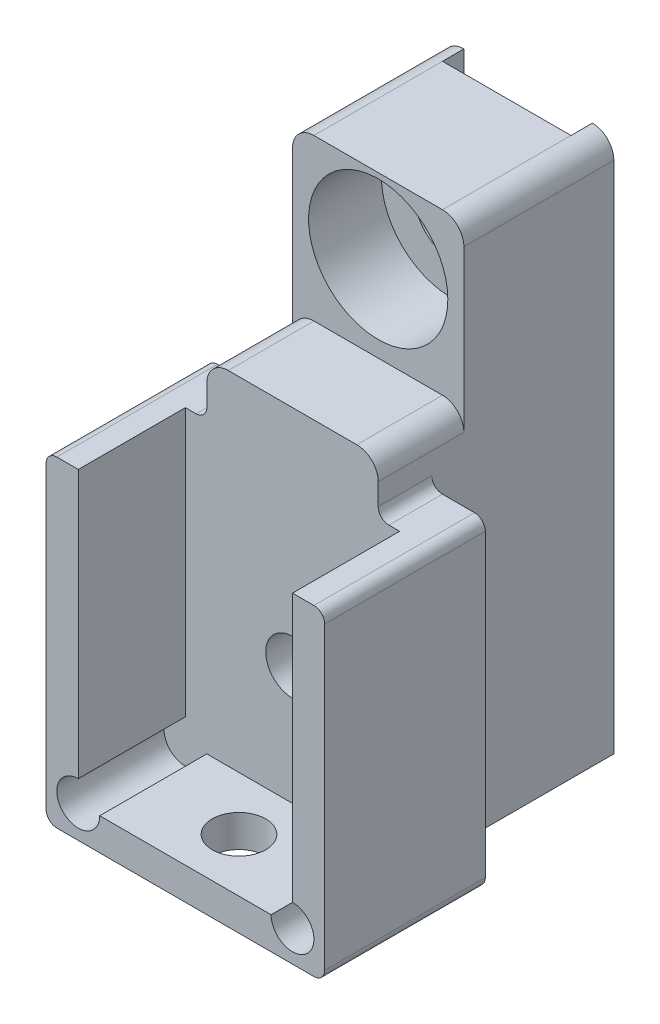
SolidWorks part; units mm, degrees
material "S136"
ref_plane "Front Plane" through (0, 0, 0) normal (0, 0, 1) x (1, 0, 0)
ref_plane "Top Plane" through (0, 0, 0) normal (0, 1, 0) x (1, 0, 0)
ref_plane "Right Plane" through (0, 0, 0) normal (1, 0, 0) x (0, 0, -1)
sketch "Sketch1" plane through (0, 0, 0) normal (0, 0, 1) x (1, 0, 0)
  line L1 (-6.5, 12.5) -> (6.5, 12.5)
  line L2 (-6.5, 12.5) -> (-6.5, -12.5)
  line L3 (-6.5, -12.5) -> (6.5, -12.5)
  line L4 (6.5, 12.5) -> (6.5, -12.5)
  line L5 (-6.5, 12.5) -> (6.5, -12.5) construction
  line L6 (-6.5, -12.5) -> (6.5, 12.5) construction
  point P0 (0, 0)
  dimension "13" = 13
  dimension "D2" = 25
extrude "Boss-Extrude1" add sketch "Sketch1" along normal blind 10
sketch "Sketch2" plane through (0, 0, 10) normal (0, 0, 1) x (1, 0, 0)
  line L0 (0, 0) -> (0, -5.4615) construction
  line L1 (-6.5, 12.5) -> (-4, 12.5)
  line L2 (-6.5, 12.5) -> (-6.5, 2.5)
  line L3 (-6.5, 2.5) -> (-4, 2.5)
  line L4 (-4, 12.5) -> (-4, 2.5)
  line L5 (4, 12.5) -> (4, 2.5)
  line L6 (6.5, 2.5) -> (4, 2.5)
  line L7 (6.5, 12.5) -> (6.5, 2.5)
  line L8 (6.5, 12.5) -> (4, 12.5)
  dimension "D1" = 4
  dimension "D2" = 10
extrude "Cut-Extrude1" cut sketch "Sketch2" against normal through all both and the other way through all
fillet "Fillet1" radius 0.5 6 edges at (4, 2.5, 5) (-4, 2.5, 5) (6.5, 2.5, 5) (6.5, -12.5, 5) (-6.5, -12.5, 5) (-6.5, 2.5, 5)
fillet "Fillet2" radius 1 2 edges at (4, 12.5, 5) (-4, 12.5, 5)
sketch "Sketch8" plane through (0, 0, 0) normal (0, 0, -1) x (-1, 0, 0)
  line L0 (-3, 12.5) -> (3, 12.5) construction
  line L1 (-3, -20.0892) -> (3, -20.0892)
  line L2 (-3, -20.0892) -> (-3, 12.5)
  line L3 (-3, 12.5) -> (3, 12.5)
  line L4 (3, -20.0892) -> (3, 12.5)
  line L5 (-3, -20.0892) -> (3, 12.5) construction
  line L6 (-3, 12.5) -> (3, -20.0892) construction
  line L7 (0, 0) -> (0, 24.6616) construction
  point P0 (0, -3.7946)
  dimension "D1" = 6
extrude "Cut-Extrude4" cut sketch "Sketch8" against normal blind 1
sketch "Sketch21" plane through (0, 0, 10) normal (0, 0, 1) x (1, 0, 0)
  line L0 (-6, -12.5) -> (6, -12.5) construction
  line L1 (-5, 19.6027) -> (5, 19.6027)
  line L2 (-5, 19.6027) -> (-5, -11)
  line L3 (-5, -11) -> (5, -11)
  line L4 (5, 19.6027) -> (5, -11)
  line L5 (6.5, -12) -> (6.5, 2) construction
  line L6 (-6.5, 2) -> (-6.5, -12) construction
  dimension "D1" = 1.5
  dimension "D2" = 1.5
  dimension "D3" = 1.5
extrude "Cut-Extrude11" cut sketch "Sketch21" against normal blind 1
sketch "Sketch25" plane through (0, 0, 9) normal (0, 0, 1) x (1, 0, 0)
  line L0 (3, 12.5) -> (-3, 12.5) construction
  line L1 (-8.1526, 20.6765) -> (5.6484, 20.6765)
  line L2 (-8.1526, 20.6765) -> (-8.1526, 5)
  line L3 (-8.1526, 5) -> (5.6484, 5)
  line L4 (5.6484, 20.6765) -> (5.6484, 5)
  dimension "D1" = 7.5
extrude "Cut-Extrude13" cut sketch "Sketch25" against normal blind 2
fillet "Fillet3" radius 1 2 edges at (4, 5, 8) (-4, 5, 8)
hole_wizard "CBORE for M3 Hex Socket Head Cap Screw2" positions "Sketch26" profile "Sketch27" counterbore size "M3" standard "ISO" end condition up to next
sketch "Sketch26" plane through (0, 0, 9) normal (0, 0, 1) x (1, 0, 0)
  line L0 (3, 12.5) -> (-3, 12.5) construction
  point P0 (0, 9)
  dimension "D2" = 3.5
sketch "Sketch27" plane through (0, 9, 9) normal (1, 0, 0) x (0, -1, 0)
  line L0 (0, 0) -> (0, 8)
  line L1 (0, 8) -> (1.7, 8)
  line L3 (1.7, 8) -> (1.7, 5.4)
  line L4 (1.7, 5.4) -> (3.25, 5.4)
  line L5 (3.25, 5.4) -> (3.25, 0)
  line L7 (3.25, 0) -> (0, 0)
  line L11 (0, -6.35) -> (0, 107.95) construction
  dimension "通孔孔直径" = 3.4
  dimension "通孔孔深度" = 8
  dimension "柱形沉头孔直径" = 6.5
  dimension "柱形沉头孔深度" = 5.4
sketch "Sketch31" plane through (0, 0, 10) normal (0, 0, 1) x (1, 0, 0)
  line L8 (-5, -11) -> (-5, 2.5)
  line L9 (-5, 2.5) -> (-6, 2.5)
  line L10 (-6.5, 2) -> (-6.5, -12)
  line L11 (-6, -12.5) -> (6, -12.5)
  line L12 (6.5, -12) -> (6.5, 2)
  line L13 (6, 2.5) -> (5, 2.5)
  line L15 (-5, -11) -> (-5, 2.5)
  line L17 (-5, 2.5) -> (-6, 2.5)
  line L18 (-6.5, 2) -> (-6.5, -12)
  line L19 (-6, -12.5) -> (6, -12.5)
  line L20 (6.5, -12) -> (6.5, 2)
  line L21 (6, 2.5) -> (5, 2.5)
  line L25 (5, 2.5) -> (5, -11)
  line L27 (5, 2.5) -> (5, -11)
  line L28 (5, -11) -> (-5, -11)
  line L29 (5, -11) -> (-5, -11)
  arc A6 (-6, 2.5) -> (-6.5, 2) centre (-6, 2) ccw
  arc A7 (-6.5, -12) -> (-6, -12.5) centre (-6, -12) ccw
  arc A8 (6, -12.5) -> (6.5, -12) centre (6, -12) ccw
  arc A9 (6.5, 2) -> (6, 2.5) centre (6, 2) ccw
  arc A12 (-6, 2.5) -> (-6.5, 2) centre (-6, 2) ccw
  arc A13 (-6.5, -12) -> (-6, -12.5) centre (-6, -12) ccw
  arc A14 (6, -12.5) -> (6.5, -12) centre (6, -12) ccw
  arc A15 (6.5, 2) -> (6, 2.5) centre (6, 2) ccw
  dimension "D1" = 0
extrude "Boss-Extrude4" add sketch "Sketch31" along normal blind 6
sketch "Sketch33" plane through (-6.5, 0, 0) normal (-1, 0, 0) x (0, 0, 1)
  line L0 (1, 12.5) -> (7, 12.5) construction
  line L1 (-1.8788, 3.5) -> (8.5, 3.5)
  line L2 (-1.8788, 3.5) -> (-1.8788, -16.5)
  line L3 (-1.8788, -16.5) -> (8.5, -16.5)
  line L4 (8.5, 3.5) -> (8.5, -16.5)
  line L5 (0, 3) -> (0, 11.5) construction
  dimension "D1" = 8.5
  dimension "D2" = 9
  dimension "D3" = 20
extrude "Cut-Extrude15" cut sketch "Sketch33" against normal up to surface (2.5 mm away) up to face at (-4, 6.1667, 5.3333)
sketch "Sketch34" plane through (6.5, 0, 0) normal (1, 0, 0) x (0, 0, -1)
  line L0 (0, -12) -> (0, 2) construction
  line L1 (-8.5, -16.2363) -> (1.421, -16.2363)
  line L2 (-8.5, -16.2363) -> (-8.5, 3.5)
  line L3 (-8.5, 3.5) -> (1.421, 3.5)
  line L4 (1.421, -16.2363) -> (1.421, 3.5)
  line L5 (-7, 12.5) -> (-1, 12.5) construction
  dimension "D1" = 8.5
  dimension "D2" = 9
extrude "Cut-Extrude16" cut sketch "Sketch34" against normal up to surface (2.5 mm away) up to face at (4, 6.1667, 5.3333)
sketch "Sketch36" plane through (0, 0, 9) normal (0, 0, 1) x (1, 0, 0)
  line L8 (-5, 2.5) -> (-5, -11)
  line L9 (-5, -11) -> (5, -11)
  line L10 (5, -11) -> (5, 2.5)
  line L11 (5, 2.5) -> (4.5, 2.5)
  line L12 (4, 3) -> (4, 4)
  line L13 (3, 5) -> (-3, 5)
  line L14 (-4, 4) -> (-4, 3)
  line L15 (-4.5, 2.5) -> (-5, 2.5)
  line L16 (-5, 2.5) -> (-5, -11)
  line L17 (-5, -11) -> (5, -11)
  line L18 (5, -11) -> (5, 2.5)
  line L19 (5, 2.5) -> (4.5, 2.5)
  line L20 (4, 3) -> (4, 4)
  line L21 (3, 5) -> (-3, 5)
  line L22 (-4, 4) -> (-4, 3)
  line L23 (-4.5, 2.5) -> (-5, 2.5)
  arc A8 (4, 3) -> (4.5, 2.5) centre (4.5, 3) ccw
  arc A9 (4, 4) -> (3, 5) centre (3, 4) ccw
  arc A10 (-3, 5) -> (-4, 4) centre (-3, 4) ccw
  arc A11 (-4.5, 2.5) -> (-4, 3) centre (-4.5, 3) ccw
  arc A14 (4, 3) -> (4.5, 2.5) centre (4.5, 3) ccw
  arc A15 (4, 4) -> (3, 5) centre (3, 4) ccw
  arc A16 (-3, 5) -> (-4, 4) centre (-3, 4) ccw
  arc A17 (-4.5, 2.5) -> (-4, 3) centre (-4.5, 3) ccw
  dimension "D1" = 0
extrude "Boss-Extrude5" add sketch "Sketch36" along normal blind 2
hole_wizard "M3 Tapped Hole1" positions "Sketch37" profile "Sketch38" tap size "M3" standard "ISO"
sketch "Sketch37" plane through (0, 0, 11) normal (0, 0, 1) x (1, 0, 0)
  line L0 (-6, -12.5) -> (6, -12.5) construction
  line L1 (6.5, -12) -> (6.5, 2) construction
  point P0 (0, -5.5)
  dimension "D1" = 7
  dimension "D2" = 6.5
sketch "Sketch38" plane through (0, -5.5, 11) normal (1, 0, 0) x (0, -1, 0)
  line L0 (0, 0) -> (0, 8.2511)
  line L1 (0, 8.2511) -> (1.25, 7.5)
  line L2 (1.25, 7.5) -> (1.25, 0)
  line L5 (1.25, 0) -> (0, 0)
  line L10 (0, 8.2511) -> (-1.25, 7.5) construction
  line L11 (0, -6.35) -> (0, 107.95) construction
  dimension "螺纹孔钻头直径" = 2.5
  dimension "螺纹孔钻头深度" = 7.5
  dimension "导头角度" = 118
cosmetic thread "Cosmetic Thread1" parameters "D1"=6, "D2"=3
hole_wizard "M3 Tapped Hole2" positions "Sketch39" profile "Sketch40" tap size "M3" standard "ISO"
sketch "Sketch39" plane through (0, -12.5, 0) normal (0, -1, 0) x (-1, 0, 0)
  line L0 (6, -16) -> (-6, -16) construction
  point P0 (0, -13.5)
  dimension "D1" = 2.5
sketch "Sketch40" plane through (0, -12.5, 13.5) normal (1, 0, 0) x (0, 0, -1)
  line L0 (0, 0) -> (0, 8.2511)
  line L1 (0, 8.2511) -> (1.25, 7.5)
  line L2 (1.25, 7.5) -> (1.25, 0)
  line L5 (1.25, 0) -> (0, 0)
  line L10 (0, 8.2511) -> (-1.25, 7.5) construction
  line L11 (0, -6.35) -> (0, 107.95) construction
  dimension "螺纹孔钻头直径" = 2.5
  dimension "螺纹孔钻头深度" = 7.5
  dimension "导头角度" = 118
cosmetic thread "Cosmetic Thread2" parameters "D1"=6, "D2"=3
sketch "Sketch41" plane through (0, 0, 16) normal (0, 0, 1) x (1, 0, 0)
  line L0 (0, 0) -> (0, -12.5) construction
  line L1 (-6, -12.5) -> (6, -12.5) construction
  circle A0 centre (-5, -11) radius 1
  circle A1 centre (5, -11) radius 1
  dimension "D1" = 2
extrude "Cut-Extrude17" cut sketch "Sketch41" against normal up to surface (5 mm away) up to face at (1.25, -5.5, 11)
